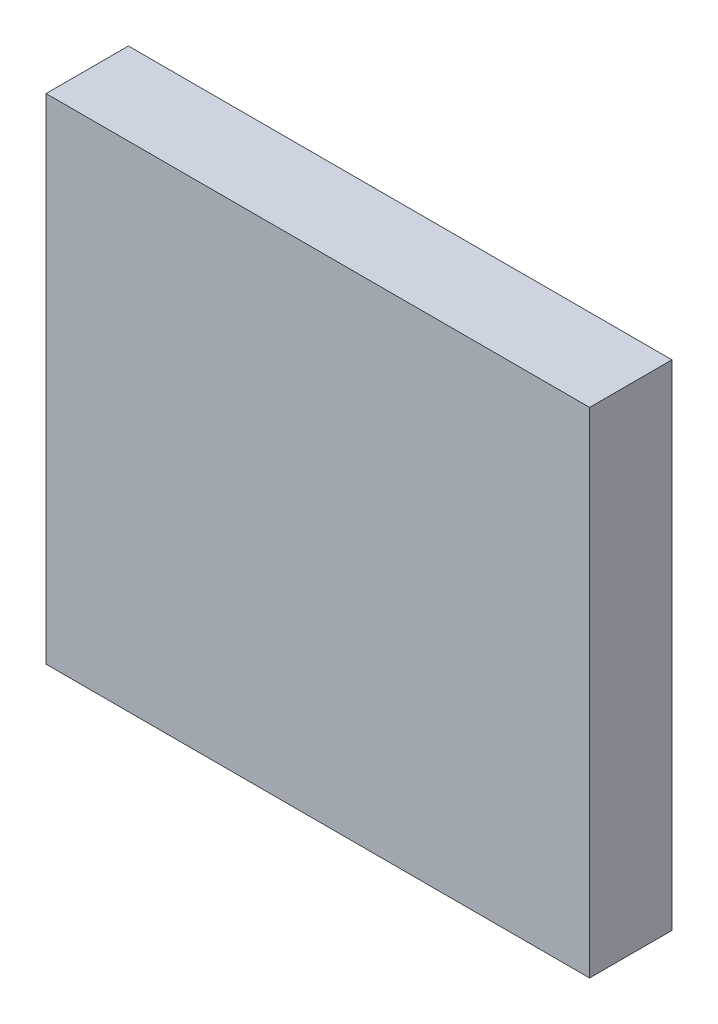
SolidWorks part; units mm, degrees
material "Q235B"
ref_plane "Front Plane" through (0, 0, 0) normal (0, 0, 1) x (1, 0, 0)
ref_plane "Top Plane" through (0, 0, 0) normal (0, 1, 0) x (1, 0, 0)
ref_plane "Right Plane" through (0, 0, 0) normal (1, 0, 0) x (0, 0, -1)
sketch "Sketch1" plane through (0, 0, 0) normal (0, 0, 1) x (1, 0, 0)
  line L1 (0, 0) -> (132, 0)
  line L2 (0, 0) -> (0, 120)
  line L3 (0, 120) -> (132, 120)
  line L4 (132, 0) -> (132, 120)
  dimension "D1" = 132
  dimension "D2" = 120
extrude "Boss-Extrude1" add sketch "Sketch1" along normal blind 20
